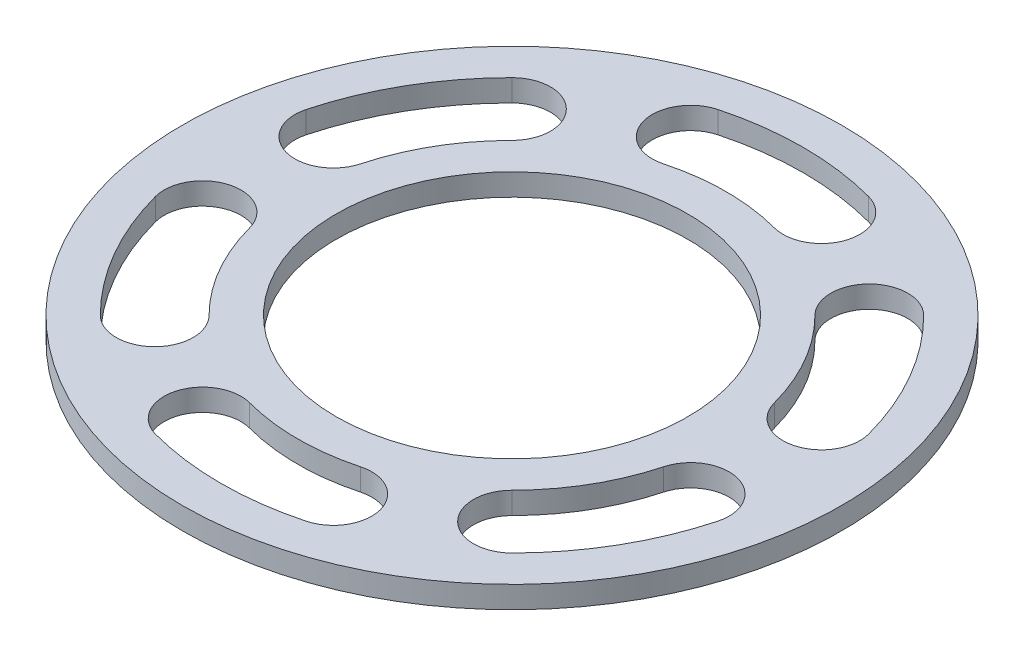
SolidWorks part; units mm, degrees
material "哈碳纤"
ref_plane "前视基准面" through (0, 0, 0) normal (0, 0, 1) x (1, 0, 0)
ref_plane "上视基准面" through (0, 0, 0) normal (0, 1, 0) x (1, 0, 0)
ref_plane "右视基准面" through (0, 0, 0) normal (1, 0, 0) x (0, 0, -1)
other "Configuration Table"
sketch "草图1" plane through (0, 0, 0) normal (0, 1, 0) x (1, 0, 0)
  circle A0 centre (0, 0) radius 16
  circle A1 centre (0, 0) radius 30
  dimension "D1" = 32
  dimension "D2" = 60
extrude "凸台-拉伸1" add sketch "草图1" along normal blind 2
sketch "草图2" plane through (0, 2, 0) normal (0, 1, 0) x (1, 0, 0)
  line L0 (-5.9528, 22.2163) -> (0, 0) construction
  line L1 (0, 0) -> (5.9528, 22.2163) construction
  line L2 (0, 23) -> (0, 0) construction
  circle A0 centre (0, 0) radius 23 construction
  arc A1 (-5.9528, 22.2163) -> (5.9528, 22.2163) centre (0, 0) cw construction
  arc A2 (6.8587, 25.597) -> (-6.8587, 25.597) centre (0, 0) ccw
  arc A3 (5.047, 18.8356) -> (-5.047, 18.8356) centre (0, 0) ccw
  arc A4 (5.047, 18.8356) -> (6.8587, 25.597) centre (5.9528, 22.2163) ccw
  arc A5 (-6.8587, 25.597) -> (-5.047, 18.8356) centre (-5.9528, 22.2163) ccw
  arc A6 (16.2635, 16.2635) -> (22.2163, 5.9528) centre (0, 0) cw construction
  arc A7 (25.597, 6.8587) -> (18.7383, 18.7383) centre (0, 0) ccw
  arc A8 (18.8356, 5.047) -> (13.7886, 13.7886) centre (0, 0) ccw
  arc A9 (18.8356, 5.047) -> (25.597, 6.8587) centre (22.2163, 5.9528) ccw
  arc A10 (18.7383, 18.7383) -> (13.7886, 13.7886) centre (16.2635, 16.2635) ccw
  arc A11 (22.2163, -5.9528) -> (16.2635, -16.2635) centre (0, 0) cw construction
  arc A12 (18.7383, -18.7383) -> (25.597, -6.8587) centre (0, 0) ccw
  arc A13 (13.7886, -13.7886) -> (18.8356, -5.047) centre (0, 0) ccw
  arc A14 (13.7886, -13.7886) -> (18.7383, -18.7383) centre (16.2635, -16.2635) ccw
  arc A15 (25.597, -6.8587) -> (18.8356, -5.047) centre (22.2163, -5.9528) ccw
  arc A16 (5.9528, -22.2163) -> (-5.9528, -22.2163) centre (0, 0) cw construction
  arc A17 (-6.8587, -25.597) -> (6.8587, -25.597) centre (0, 0) ccw
  arc A18 (-5.047, -18.8356) -> (5.047, -18.8356) centre (0, 0) ccw
  arc A19 (-5.047, -18.8356) -> (-6.8587, -25.597) centre (-5.9528, -22.2163) ccw
  arc A20 (6.8587, -25.597) -> (5.047, -18.8356) centre (5.9528, -22.2163) ccw
  arc A21 (-16.2635, -16.2635) -> (-22.2163, -5.9528) centre (0, 0) cw construction
  arc A22 (-25.597, -6.8587) -> (-18.7383, -18.7383) centre (0, 0) ccw
  arc A23 (-18.8356, -5.047) -> (-13.7886, -13.7886) centre (0, 0) ccw
  arc A24 (-18.8356, -5.047) -> (-25.597, -6.8587) centre (-22.2163, -5.9528) ccw
  arc A25 (-18.7383, -18.7383) -> (-13.7886, -13.7886) centre (-16.2635, -16.2635) ccw
  arc A26 (-22.2163, 5.9528) -> (-16.2635, 16.2635) centre (0, 0) cw construction
  arc A27 (-18.7383, 18.7383) -> (-25.597, 6.8587) centre (0, 0) ccw
  arc A28 (-13.7886, 13.7886) -> (-18.8356, 5.047) centre (0, 0) ccw
  arc A29 (-13.7886, 13.7886) -> (-18.7383, 18.7383) centre (-16.2635, 16.2635) ccw
  arc A30 (-25.597, 6.8587) -> (-18.8356, 5.047) centre (-22.2163, 5.9528) ccw
  point P5 (0, 23)
  point P20 (19.9186, 11.5)
  point P27 (19.9186, -11.5)
  point P34 (0, -23)
  point P41 (-19.9186, -11.5)
  point P48 (-19.9186, 11.5)
  point P53 (0, 0)
  dimension "D1" = 46
  dimension "D2" = 30
  dimension "D3" = 7
  dimension "D4" = 6
extrude "切除-拉伸1" cut sketch "草图2" against normal through all both and the other way through all
